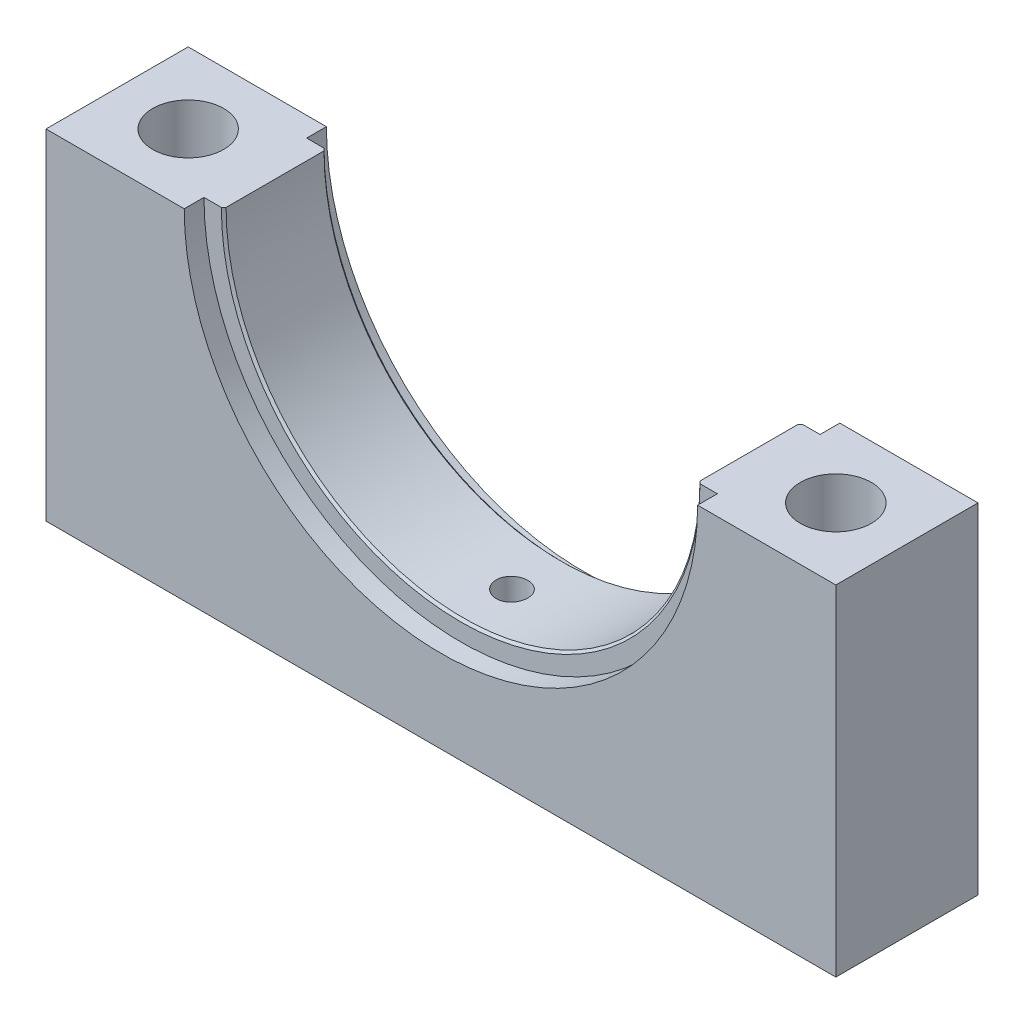
from build123d import *

# Parameters (mm, degrees)
BOSS_EXTRUDE1_DEPTH = 18
SKETCH2_R           = 32.5
CUT_EXTRUDE1_DEPTH  = 2.5
CUT_EXTRUDE2_START  = -2.5
SKETCH3_R           = 32.5
CUT_EXTRUDE2_DEPTH  = 2.5
CHAMFER1_SIZE       = 0.3
HOLE1_D             = 9
HOLE2_D             = 4
HOLE2_DEPTH         = 34


with BuildPart() as part:
    # Sketch1 → Boss-Extrude1 (new body)
    with BuildSketch(Plane.XY):
        with BuildLine():
            Line((-50, 0), (-30, 0))
            ThreePointArc((-30, 0), (0, -30), (30, 0))
            Line((30, 0), (50, 0))
            Line((50, 0), (50, -43))
            Line((50, -43), (-50, -43))
            Line((-50, -43), (-50, 0))
        make_face()
    extrude(amount=BOSS_EXTRUDE1_DEPTH)

    # Sketch2 → Cut-Extrude1 (cut)
    with BuildSketch(Plane.XY.offset(18)):
        Circle(SKETCH2_R)
    extrude(amount=-CUT_EXTRUDE1_DEPTH, mode=Mode.SUBTRACT)

    # Sketch3 → Cut-Extrude2 (cut)
    with BuildSketch(Plane(origin=(0, 0, 0), x_dir=(-1, 0, 0), z_dir=(0, 0, -1)).offset(CUT_EXTRUDE2_START)):
        Circle(SKETCH3_R)
    extrude(amount=CUT_EXTRUDE2_DEPTH, mode=Mode.SUBTRACT)

    # Chamfer1
    chamfer1_edges = [part.edges().sort_by_distance(p)[0] for p in [
        (0, -30, 15.5),
        (0, -30, 2.5),
    ]]
    chamfer(chamfer1_edges, length=CHAMFER1_SIZE)

    # Hole1 (through all)
    with Locations(Plane(origin=(0, 0, 0), x_dir=(1, 0, 0), z_dir=(0, 1, 0))):
        with Locations((-41, -9), (41, -9)):
            Hole(HOLE1_D / 2)

    # Hole2
    with Locations(Plane(origin=(0, 0, 0), x_dir=(1, 0, 0), z_dir=(0, 1, 0))):
        with Locations((0, -9)):
            Hole(HOLE2_D / 2, depth=HOLE2_DEPTH)


solid = part.part
